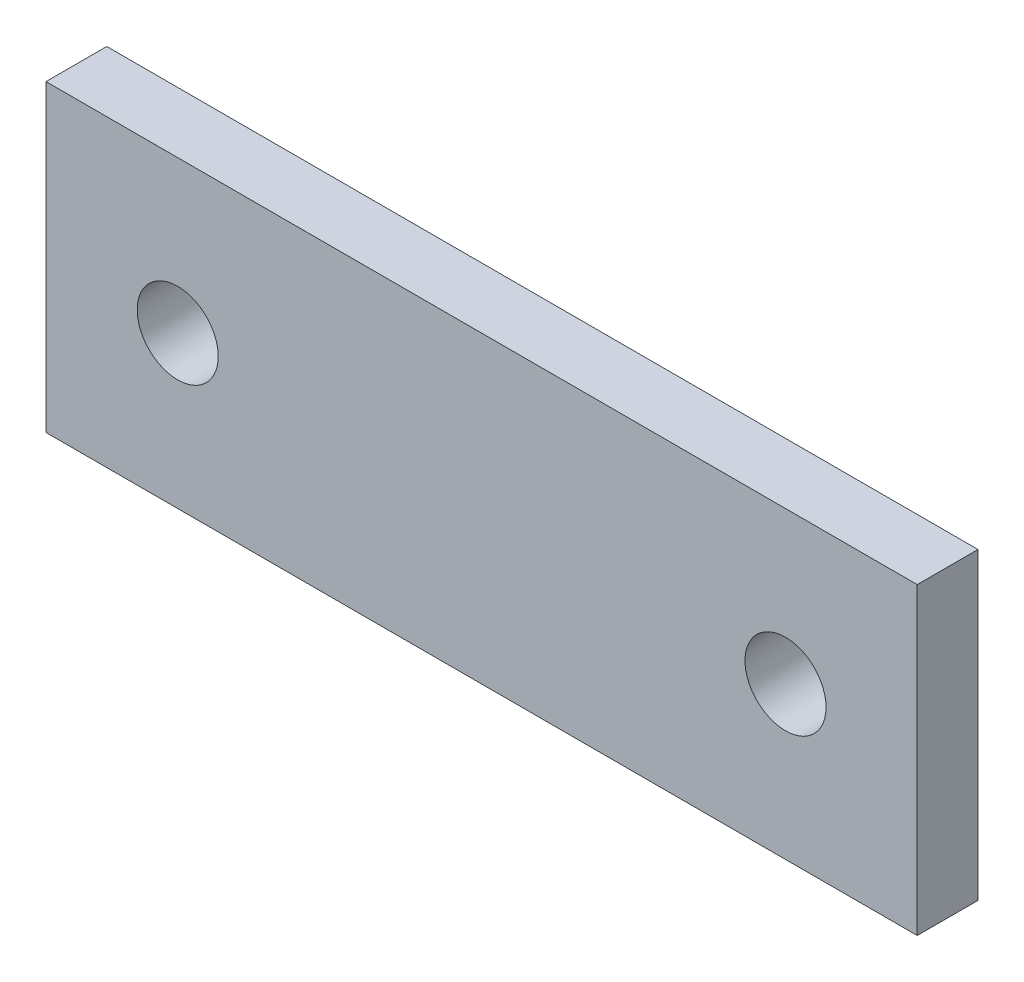
from build123d import *

# Parameters (mm, degrees)
SKETCH1_W           = 86
SKETCH1_H           = 30
BOSS_EXTRUDE1_DEPTH = 6
SKETCH2_R           = 4
CUT_EXTRUDE1_DEPTH  = 10


with BuildPart() as part:
    # Sketch1 → Boss-Extrude1 (new body)
    with BuildSketch(Plane.XY):
        Rectangle(SKETCH1_W, SKETCH1_H)
    extrude(amount=BOSS_EXTRUDE1_DEPTH)

    # Sketch2 → Cut-Extrude1 (cut)
    with BuildSketch(Plane.XY.offset(6)):
        with Locations((-30, 0)):
            Circle(SKETCH2_R)
        with Locations((30, 0)):
            Circle(SKETCH2_R)
    extrude(amount=-CUT_EXTRUDE1_DEPTH, mode=Mode.SUBTRACT)


solid = part.part
